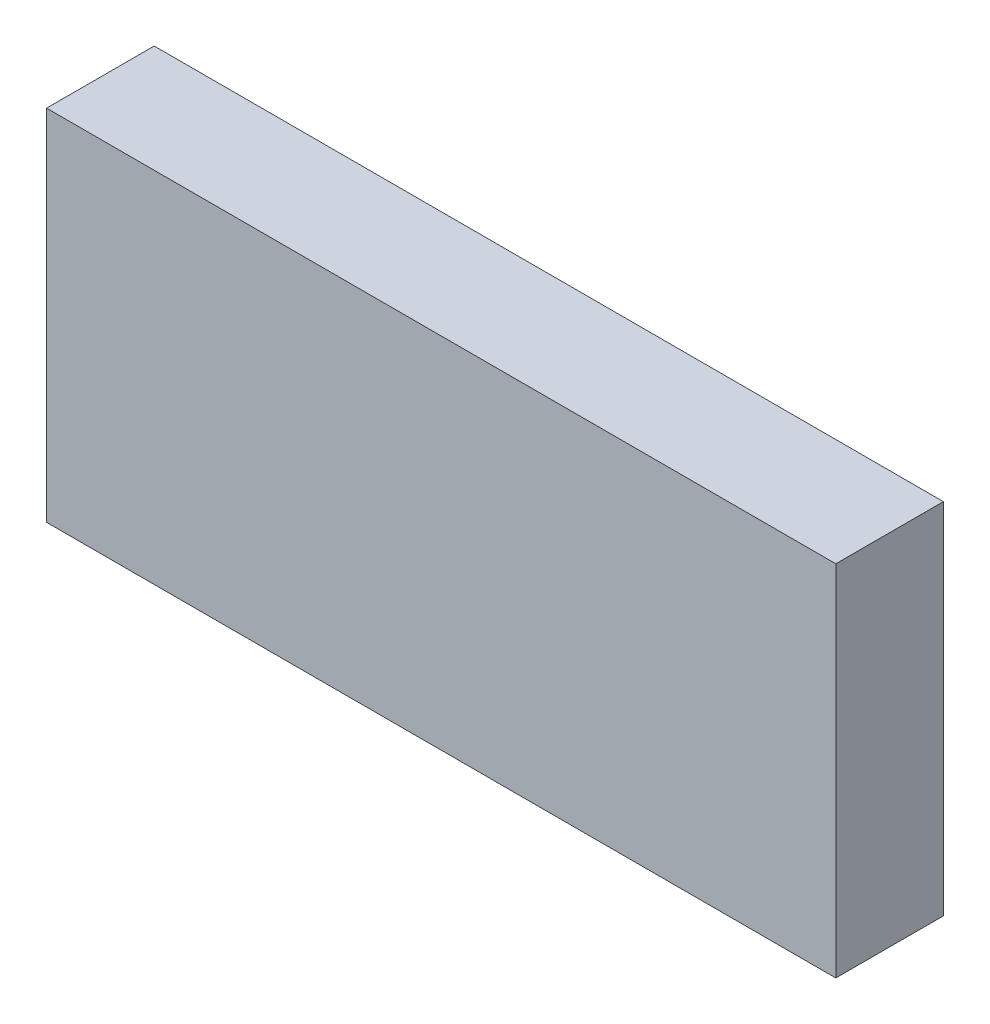
SolidWorks part; units mm, degrees
ref_plane "Front Plane" through (0, 0, 0) normal (0, 0, 1) x (1, 0, 0)
ref_plane "Top Plane" through (0, 0, 0) normal (0, 1, 0) x (1, 0, 0)
ref_plane "Right Plane" through (0, 0, 0) normal (1, 0, 0) x (0, 0, -1)
sketch "Sketch1" plane through (0, 0, 0) normal (0, 1, 0) x (1, 0, 0)
  line L1 (-110, -15) -> (110, -15)
  line L2 (-110, -15) -> (-110, 15)
  line L3 (-110, 15) -> (110, 15)
  line L4 (110, -15) -> (110, 15)
  line L5 (-110, -15) -> (110, 15) construction
  line L6 (-110, 15) -> (110, -15) construction
  point P0 (0, 0)
  dimension "D1" = 30
  dimension "D2" = 220
extrude "Boss-Extrude1" add sketch "Sketch1" along normal blind 100
